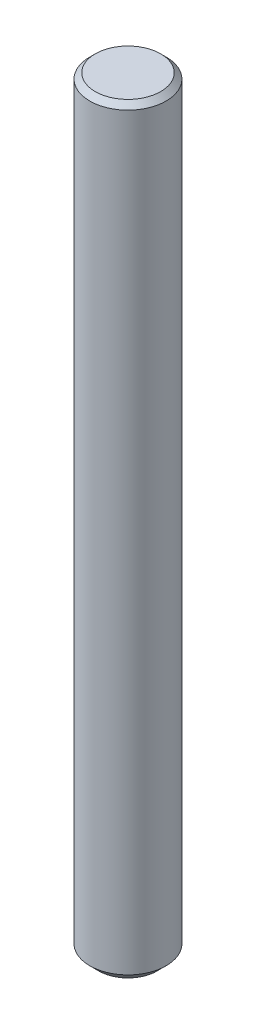
SolidWorks part; units mm, degrees
material "普通碳钢"
ref_plane "Front Plane" through (0, 0, 0) normal (0, 0, 1) x (1, 0, 0)
ref_plane "Top Plane" through (0, 0, 0) normal (0, 1, 0) x (1, 0, 0)
ref_plane "Right Plane" through (0, 0, 0) normal (1, 0, 0) x (0, 0, -1)
sketch "Sketch2" plane through (0, 0, 0) normal (0, 1, 0) x (1, 0, 0)
  circle A0 centre (0, 0) radius 21
  dimension "D1" = 42
extrude "Boss-Extrude1" add sketch "Sketch2" along normal blind 420
chamfer "Chamfer1" distance 5 angle 45 1 edges at (0, 0, 21)
chamfer "Chamfer2" distance 3 angle 45 1 edges at (0, 420, 21)
